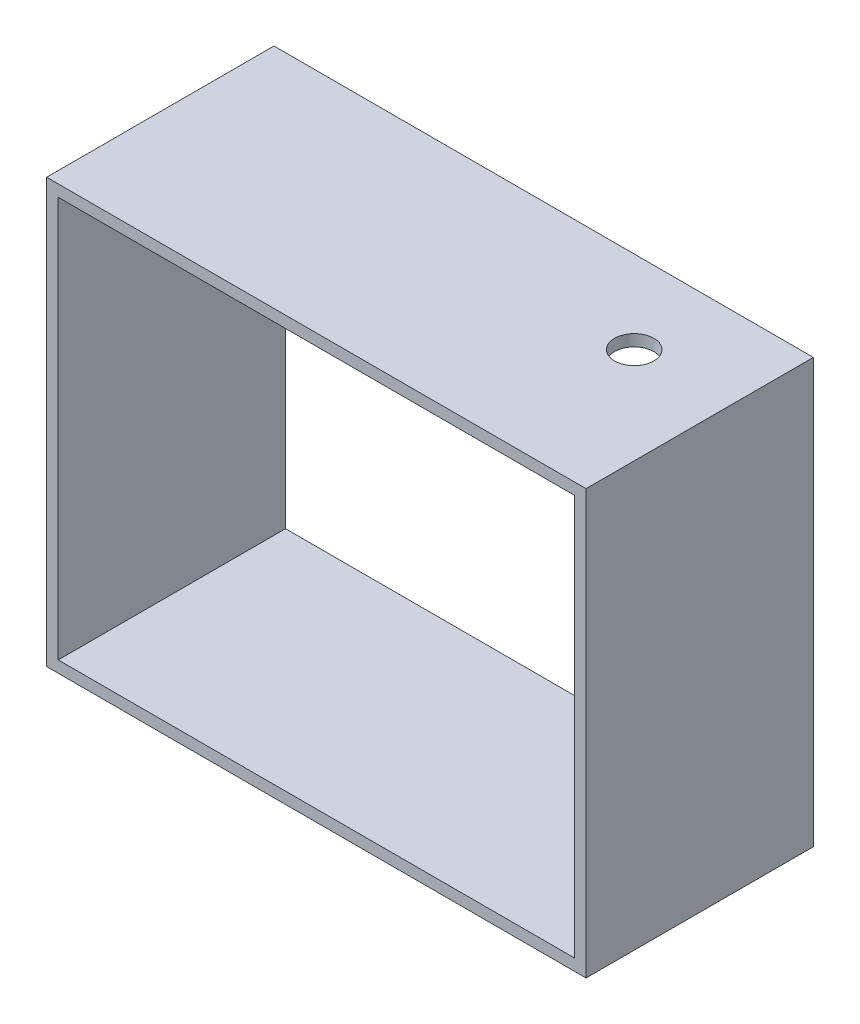
from build123d import *

# Parameters (mm, degrees)
SKETCH_1_W          = 140
SKETCH_1_H          = 110
SKETCH_1_W_2        = 134
SKETCH_1_H_2        = 104
EXTRUDE_1_DEPTH     = 29.5
SKETCH_2_R          = 5.1
CUT_EXTRUDE_1_DEPTH = 70


with BuildPart() as part:
    # 草图1 → 凸台-拉伸1 (new, symmetric)
    with BuildSketch(Plane.XY):
        Rectangle(SKETCH_1_W, SKETCH_1_H)
        Rectangle(SKETCH_1_W_2, SKETCH_1_H_2, mode=Mode.SUBTRACT)
    extrude(amount=EXTRUDE_1_DEPTH, both=True)

    # 草图2 → 切除-拉伸1 (cut, symmetric)
    with BuildSketch(Plane(origin=(0, 0, 0), x_dir=(1, 0, 0), z_dir=(0, 1, 0))):
        with Locations(Location((45, 8, 0), (0, 0, 90))):
            Circle(SKETCH_2_R)
    extrude(amount=CUT_EXTRUDE_1_DEPTH, both=True, mode=Mode.SUBTRACT)


solid = part.part
